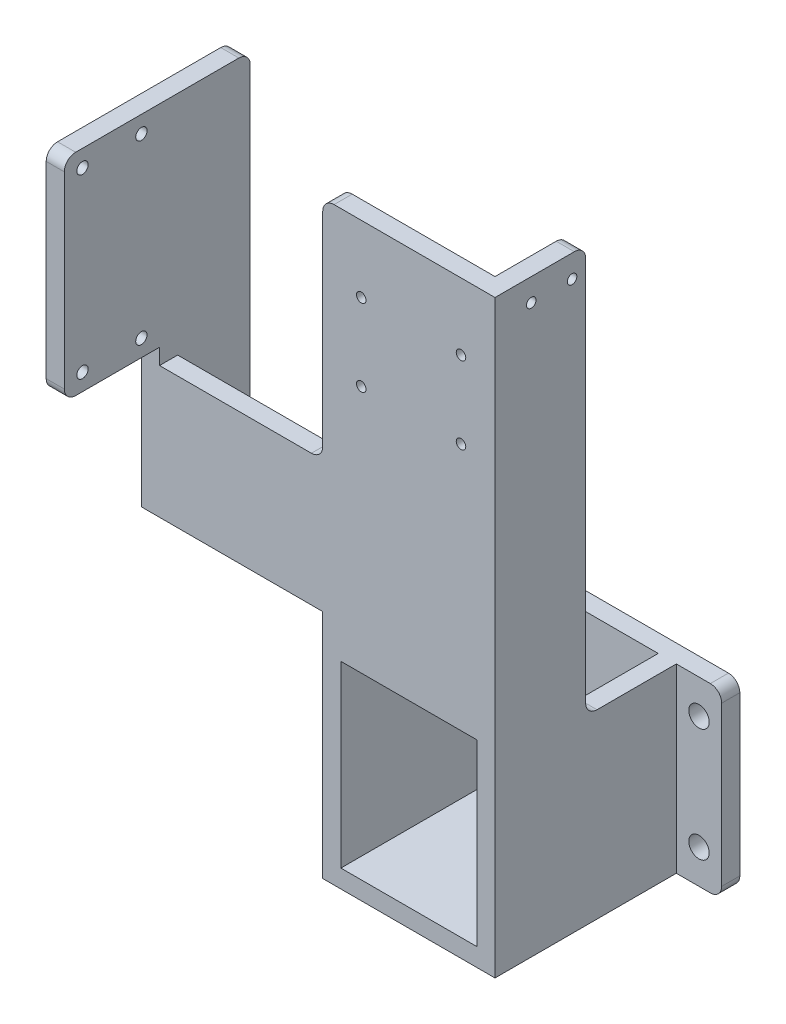
SolidWorks part; units mm, degrees
ref_plane "前视基准面" through (0, 0, 0) normal (0, 0, 1) x (1, 0, 0)
ref_plane "上视基准面" through (0, 0, 0) normal (0, 1, 0) x (1, 0, 0)
ref_plane "右视基准面" through (0, 0, 0) normal (1, 0, 0) x (0, 0, -1)
sketch "草图1" plane through (0, 0, 0) normal (0, 0, 1) x (1, 0, 0)
  line L1 (0, 0) -> (116, 0)
  line L2 (0, 0) -> (0, 80)
  line L3 (0, 80) -> (116, 80)
  line L4 (116, 0) -> (116, 80)
  dimension "D1" = 116
  dimension "D2" = 80
extrude "凸台-拉伸1" add sketch "草图1" along normal blind 8
sketch "草图2" plane through (0, 0, 8) normal (0, 0, 1) x (1, 0, 0)
  line L0 (116, 80) -> (0, 80) construction
  line L1 (20, 80) -> (28, 80)
  line L2 (20, 80) -> (20, 0)
  line L3 (20, 0) -> (28, 0)
  line L4 (28, 80) -> (28, 0)
  line L5 (0, 0) -> (116, 0) construction
  line L6 (58, 80) -> (58, 0) construction
  line L8 (88, 80) -> (96, 80)
  line L9 (88, 80) -> (88, 0)
  line L10 (88, 0) -> (96, 0)
  line L11 (96, 80) -> (96, 0)
  dimension "D1" = 8
  dimension "D2" = 60
extrude "凸台-拉伸2" add sketch "草图2" along normal blind 80
sketch "草图4" plane through (0, 80, 0) normal (0, 1, 0) x (1, 0, 0)
  line L0 (88, -88) -> (88, -8) construction
  line L1 (96, -88) -> (88, -88)
  line L2 (96, -88) -> (96, -48)
  line L3 (96, -48) -> (88, -48)
  line L4 (88, -88) -> (88, -48)
  dimension "D1" = 40
extrude "凸台-拉伸3" add sketch "草图4" along normal blind 180
sketch "草图5" plane through (0, 0, 8) normal (0, 0, 1) x (1, 0, 0)
  line L0 (28, 0) -> (28, 80) construction
  line L1 (88, 0) -> (28, 0)
  line L2 (88, 0) -> (88, 8)
  line L3 (88, 8) -> (28, 8)
  line L4 (28, 0) -> (28, 8)
  dimension "D1" = 8
extrude "凸台-拉伸4" add sketch "草图5" along normal blind 80
sketch "草图8" plane through (0, 80, 0) normal (0, 1, 0) x (1, 0, 0)
  line L1 (28, -88) -> (20, -88)
  line L2 (28, -88) -> (28, -48)
  line L3 (28, -48) -> (20, -48)
  line L4 (20, -88) -> (20, -48)
  line L5 (20, -88) -> (20, -8) construction
  dimension "D1" = 40
extrude "凸台-拉伸7" add sketch "草图8" along normal blind 30
sketch "草图10" plane through (20, 0, 0) normal (-1, 0, 0) x (0, 0, 1)
  line L0 (48, 110) -> (48, 80) construction
  line L1 (88, 110) -> (48, 110)
  line L2 (88, 110) -> (88, 102)
  line L3 (88, 102) -> (48, 102)
  line L4 (48, 110) -> (48, 102)
  dimension "D1" = 8
extrude "凸台-拉伸8" add sketch "草图10" along normal blind 80
sketch "草图11" plane through (0, 110, 0) normal (0, 1, 0) x (1, 0, 0)
  line L0 (28, -48) -> (-60, -48) construction
  line L1 (-60, -88) -> (-52, -88)
  line L2 (-60, -88) -> (-60, -48)
  line L3 (-60, -48) -> (-52, -48)
  line L4 (-52, -88) -> (-52, -48)
  dimension "D1" = 8
extrude "凸台-拉伸9" add sketch "草图11" along normal up to surface (150 mm away) up to face at (92, 260, 68)
sketch "草图12" plane through (88, 0, 0) normal (-1, 0, 0) x (0, 0, 1)
  line L1 (88, 260) -> (80, 260)
  line L2 (88, 260) -> (88, 167)
  line L3 (88, 167) -> (80, 167)
  line L4 (80, 260) -> (80, 167)
  dimension "D1" = 93
  dimension "D2" = 8
extrude "凸台-拉伸10" add sketch "草图12" along normal blind 68
sketch "草图14" plane through (0, 0, 88) normal (0, 0, 1) x (1, 0, 0)
  line L0 (-52, 260) -> (-52, 110) construction
  line L1 (-60, 260) -> (-52, 260)
  line L2 (-60, 260) -> (-60, 167)
  line L3 (-60, 167) -> (-52, 167)
  line L4 (-52, 260) -> (-52, 167)
  dimension "D1" = 93
extrude "凸台-拉伸12" add sketch "草图14" along normal blind 42
fillet "圆角1" radius 5 7 edges at (-56, 260, 48) (24, 80, 48) (92, 260, 48) (-56, 260, 130) (-56, 167, 130) (20, 260, 84)
fillet "圆角2" radius 5 4 edges at (0, 80, 4) (0, 0, 4) (116, 80, 4) (116, 0, 4)
hole_wizard "Ø9.0 (9) 直径孔1" positions "草图16" profile "草图15" hole size "Ø9.0" standard "GB" end condition through all
sketch "草图16" plane through (0, 0, 8) normal (0, 0, 1) x (1, 0, 0)
  line L3 (96, 40) -> (116, 40) construction
  line L4 (96, 0) -> (96, 80) construction
  line L5 (116, 5) -> (116, 75) construction
  point P0 (106, 15)
  point P2 (106, 65)
  dimension "D1" = 50
  dimension "D2" = 10
sketch "草图15" plane through (106, 15, 8) normal (1, 0, 0) x (0, -1, 0)
  line L0 (0, 0) -> (0, 8)
  line L1 (0, 8) -> (4.5, 8)
  line L2 (4.5, 8) -> (4.5, 0)
  line L5 (4.5, 0) -> (0, 0)
  line L11 (0, -6.35) -> (0, 107.95) construction
  dimension "通孔孔直径" = 9
  dimension "通孔孔深度" = 8
ref_plane "基准面1" through (58, 0, 0) normal (1, 0, 0) x (0, 0, -1)
mirror "镜向1" about plane through (58, 0, 0) normal (1, 0, 0) of "Ø9.0 (9) 直径孔1"
hole_wizard "M5 螺纹孔1" positions "草图18" profile "草图17" tap size "M5" standard "ISO" end condition through all
sketch "草图18" plane through (0, 0, 88) normal (0, 0, 1) x (1, 0, 0)
  point P0 (37, 196.5)
  point P3 (81, 196.5)
  point P6 (81, 230.5)
  point P9 (37, 230.5)
sketch "草图17" plane through (37, 196.5, 88) normal (1, 0, 0) x (0, -1, 0)
  line L0 (0, 0) -> (0, 88)
  line L1 (0, 88) -> (2.1, 88)
  line L2 (2.1, 88) -> (2.1, 0)
  line L5 (2.1, 0) -> (0, 0)
  line L11 (0, -6.35) -> (0, 107.95) construction
  dimension "通孔螺纹孔钻头直径" = 4.2
  dimension "通孔螺纹孔钻头深度" = 88
cosmetic thread "孔螺蚊线1" parameters "D2"=5
cosmetic thread "孔螺蚊线2" parameters "D2"=5
cosmetic thread "孔螺蚊线3" parameters "D2"=5
cosmetic thread "孔螺蚊线4" parameters "D2"=5
hole_wizard "M6 螺纹孔1" positions "草图20" profile "草图19" tap size "M6" standard "ISO" end condition through all
sketch "草图20" plane through (-52, 0, 0) normal (1, 0, 0) x (0, 0, -1)
  point P0 (-96, 252.5)
  point P3 (-122, 252.5)
  point P6 (-122, 174.5)
  point P9 (-96, 174.5)
sketch "草图19" plane through (-52, 252.5, 96) normal (0, 1, 0) x (0, 0, -1)
  line L0 (0, 0) -> (0, 8.0001)
  line L1 (0, 8.0001) -> (2.5, 8.0001)
  line L2 (2.5, 8.0001) -> (2.5, 0)
  line L5 (2.5, 0) -> (0, 0)
  line L11 (0, -6.35) -> (0, 107.95) construction
  dimension "通孔螺纹孔钻头直径" = 5
  dimension "通孔螺纹孔钻头深度" = 8.0001
cosmetic thread "孔螺蚊线5" parameters "D2"=6
cosmetic thread "孔螺蚊线6" parameters "D2"=6
cosmetic thread "孔螺蚊线7" parameters "D2"=6
cosmetic thread "孔螺蚊线8" parameters "D2"=6
hole_wizard "M5 螺纹孔2" positions "草图22" profile "草图21" tap size "M5" standard "ISO"
sketch "草图22" plane through (96, 0, 0) normal (1, 0, 0) x (0, 0, -1)
  point P0 (-72, 250)
  point P3 (-54, 250)
cosmetic thread "孔螺蚊线9" parameters "D1"=8, "D2"=5
cosmetic thread "孔螺蚊线10" parameters "D1"=8, "D2"=5
sketch "草图21" plane through (96, 250, 72) normal (0, 1, 0) x (0, 0, -1)
  line L0 (0, 0) -> (0, 11.6618)
  line L1 (0, 11.6618) -> (2.1, 10.4)
  line L2 (2.1, 10.4) -> (2.1, 0)
  line L5 (2.1, 0) -> (0, 0)
  line L10 (0, 11.6618) -> (-2.1, 10.4) construction
  line L11 (0, -6.35) -> (0, 107.95) construction
  dimension "螺纹孔钻头直径" = 4.2
  dimension "螺纹孔钻头深度" = 10.4
  dimension "导头角度" = 118
sketch "草图27" plane through (0, 0, 88) normal (0, 0, 1) x (1, 0, 0)
  line L1 (28, 8) -> (28, 110) construction
  line L2 (88, 167) -> (28, 167)
  line L3 (88, 167) -> (88, 87)
  line L4 (88, 87) -> (28, 87)
  line L5 (28, 167) -> (28, 87)
  line L7 (28, 110) -> (-52, 110)
  line L8 (28, 110) -> (28, 160)
  line L9 (28, 160) -> (-52, 160)
  line L10 (-52, 110) -> (-52, 160)
  line L11 (-52, 167) -> (-52, 110) construction
  line L13 (28, 160) -> (20, 160)
  line L14 (28, 160) -> (28, 167)
  line L15 (28, 167) -> (20, 167)
  line L16 (20, 160) -> (20, 167)
  dimension "D1" = 80
  dimension "D2" = 50
extrude "凸台-拉伸15" add sketch "草图27" against normal blind 8
fillet "圆角3" radius 5 1 edges at (20, 160, 84)
